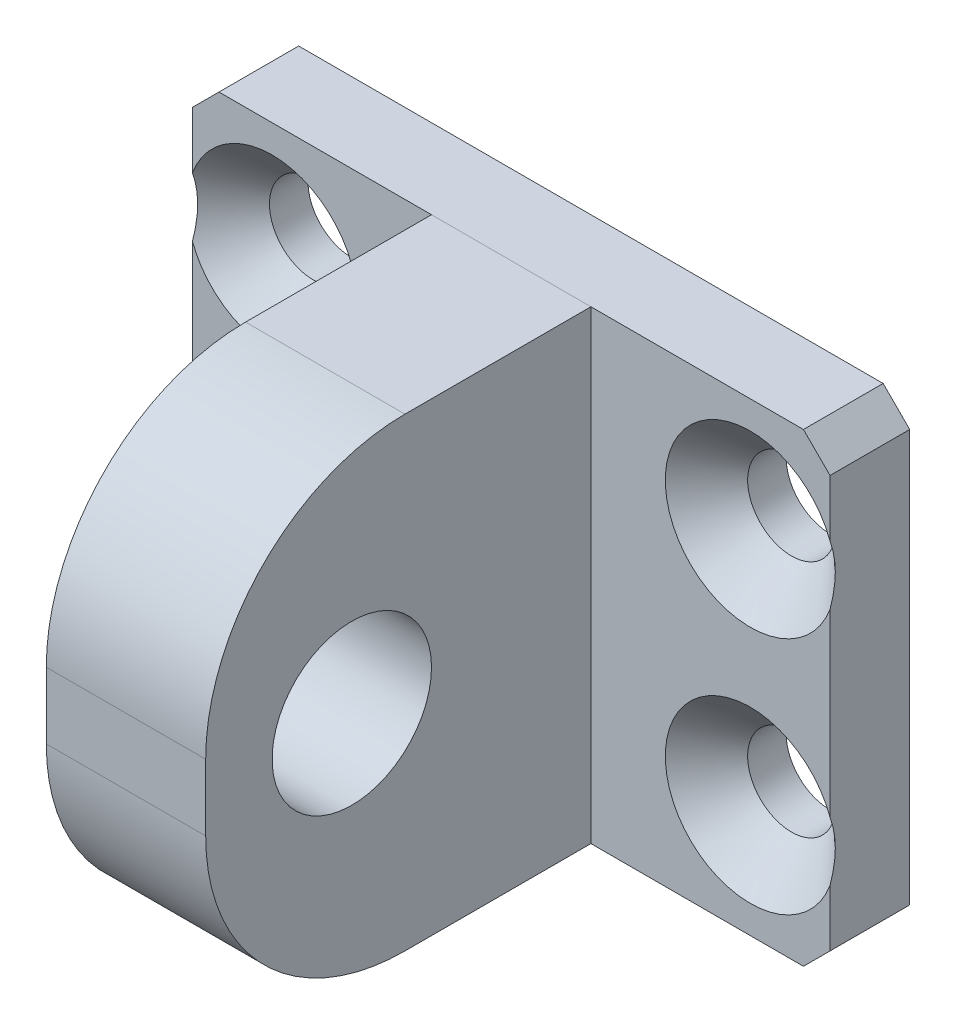
SolidWorks part; units mm, degrees
material "橡胶"
ref_plane "Front Plane" through (0, 0, 0) normal (0, 0, 1) x (1, 0, 0)
ref_plane "Top Plane" through (0, 0, 0) normal (0, 1, 0) x (1, 0, 0)
ref_plane "Right Plane" through (0, 0, 0) normal (1, 0, 0) x (0, 0, -1)
sketch "Sketch1" plane through (0, 0, 0) normal (0, 0, 1) x (1, 0, 0)
  line L1 (-24, 17.5) -> (24, 17.5)
  line L2 (-24, 17.5) -> (-24, -17.5)
  line L3 (-24, -17.5) -> (24, -17.5)
  line L4 (24, 17.5) -> (24, -17.5)
  line L5 (-24, 17.5) -> (24, -17.5) construction
  line L6 (-24, -17.5) -> (24, 17.5) construction
  point P0 (0, 0)
  dimension "D1" = 48
  dimension "D2" = 35
extrude "Boss-Extrude1" add sketch "Sketch1" along normal blind 6
sketch "Sketch2" plane through (0, 0, 6) normal (0, 0, 1) x (1, 0, 0)
  line L1 (-6, 17.5) -> (6, 17.5)
  line L2 (-6, 17.5) -> (-6, -17.5)
  line L3 (-6, -17.5) -> (6, -17.5)
  line L4 (6, 17.5) -> (6, -17.5)
  line L5 (-6, 17.5) -> (6, -17.5) construction
  line L6 (-6, -17.5) -> (6, 17.5) construction
  point P0 (0, 0)
  dimension "D1" = 12
  dimension "D2" = 35
extrude "Boss-Extrude2" add sketch "Sketch2" along normal blind 29 separate body
fillet "Fillet1" radius 15 2 edges at (0, -17.5, 35) (0, 17.5, 35)
sketch "Sketch3" plane through (6, 0, 0) normal (1, 0, 0) x (0, 0, -1)
  line L0 (-24, 0) -> (0, 0) construction
  line L1 (0, -17.5) -> (0, 17.5) construction
  circle A0 centre (-24, 0) radius 6
  dimension "D1" = 12
  dimension "D2" = 24
extrude "Cut-Extrude1" cut sketch "Sketch3" against normal blind 20
chamfer "Chamfer1" distance 2 angle 45 4 edges at (24, 17.5, 3) (24, -17.5, 3) (-24, -17.5, 3) (-24, 17.5, 3)
hole_wizard "Hole Size slotted raised countersunk screw type 1" positions "Sketch4" profile "Sketch5" countersink size "M6" standard "GB" end condition through all
sketch "Sketch4" plane through (0, 0, 6) normal (0, 0, 1) x (1, 0, 0)
  line L0 (0, 17.5) -> (0, 12.9873) construction
  line L1 (-6, 17.5) -> (6, 17.5) construction
  line L3 (0, 0) -> (24, 0) construction
  line L4 (24, -15.5) -> (24, 15.5) construction
  point P0 (-18, 9)
  point P2 (-18, -9)
  point P4 (18, 9)
  point P6 (18, -9)
  dimension "D1" = 36
  dimension "D2" = 18
sketch "Sketch5" plane through (-18, 9, 6) normal (1, 0, 0) x (0, -1, 0)
  line L0 (0, 0) -> (0, 6)
  line L1 (0, 6) -> (3.3, 6)
  line L2 (3.3, 6) -> (3.3, 3.1)
  line L3 (3.3, 3.1) -> (6.4, 0)
  line L5 (6.4, 0) -> (0, 0)
  line L6 (-3.3, 3.1) -> (-6.4, 0) construction
  line L11 (0, -6.35) -> (0, 107.95) construction
  dimension "通孔孔直径" = 6.6
  dimension "通孔孔深度" = 6
  dimension "近端锥形沉头孔直径" = 12.8
  dimension "近端锥形沉头孔角度" = 90
